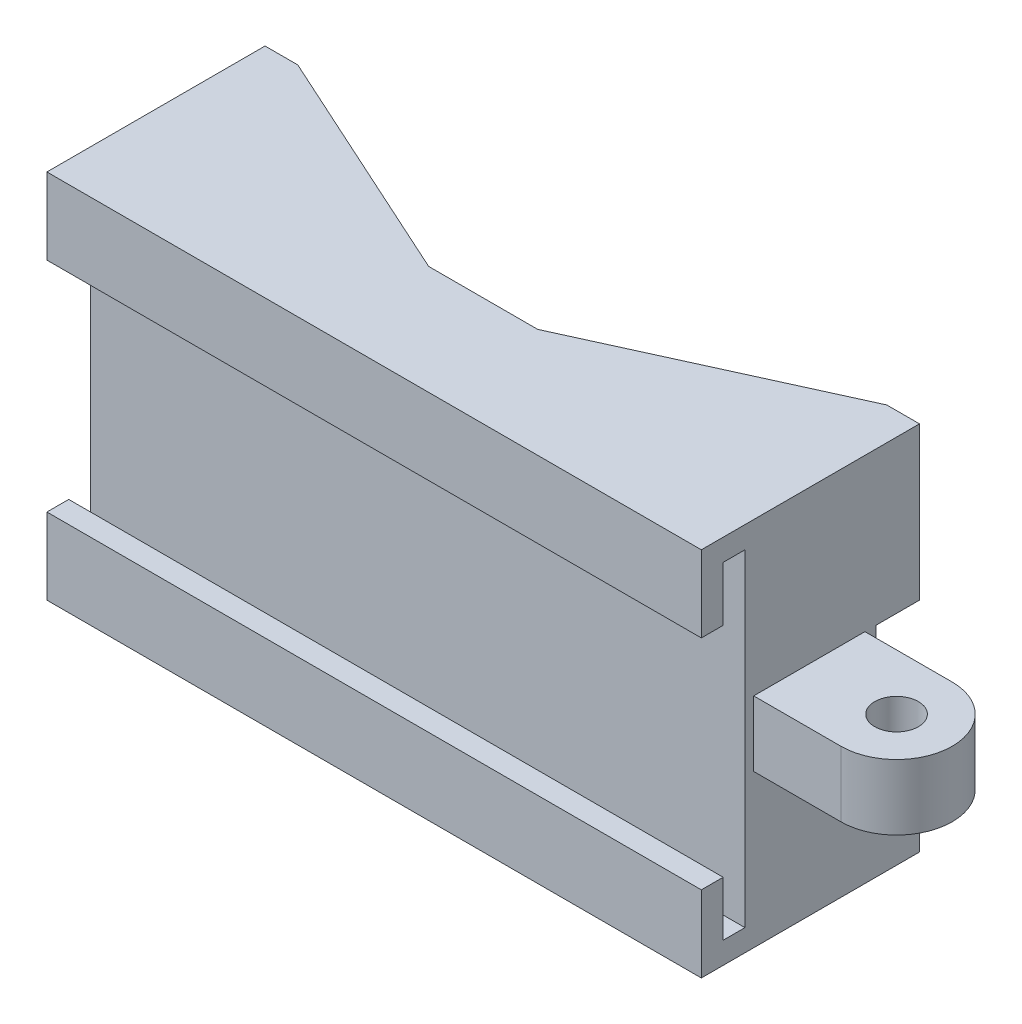
from build123d import *

# Parameters (mm, degrees)
SKETCH1_W           = 300
SKETCH1_H           = 170
BOSS_EXTRUDE1_DEPTH = 10
SKETCH2_W           = 300
SKETCH2_H           = 10
BOSS_EXTRUDE2_DEPTH = 20
SKETCH4_W           = 300
SKETCH4_H           = 10
BOSS_EXTRUDE3_DEPTH = 25
BOSS_EXTRUDE4_DEPTH = 85
CUT_EXTRUDE1_DEPTH  = 15
SKETCH8_R           = 10
BOSS_EXTRUDE5_DEPTH = 15


with BuildPart() as part:
    # Sketch1 → Boss-Extrude1 (new body)
    with BuildSketch(Plane.XY):
        Rectangle(SKETCH1_W, SKETCH1_H)
    extrude(amount=BOSS_EXTRUDE1_DEPTH)

    # Sketch2 → Boss-Extrude2 (add)
    with BuildSketch(Plane.XY.offset(10)):
        with Locations((0, 80)):
            Rectangle(SKETCH2_W, SKETCH2_H)
        with Locations((0, -80)):
            Rectangle(SKETCH2_W, SKETCH2_H)
    extrude(amount=BOSS_EXTRUDE2_DEPTH)

    # Sketch4 → Boss-Extrude3 (add)
    with BuildSketch(Plane.XZ.offset(-75)):
        with Locations((0, 25)):
            Rectangle(SKETCH4_W, SKETCH4_H)
    boss_extrude3 = extrude(amount=BOSS_EXTRUDE3_DEPTH)

    # Mirror1: Boss-Extrude3 across plane
    add(boss_extrude3.mirror(Plane.ZX))

    # Sketch5 → Boss-Extrude4 (add, symmetric)
    with BuildSketch(Plane(origin=(0, 0, 0), x_dir=(1, 0, 0), z_dir=(0, 1, 0))):
        Polygon((-150, 0), (-150, 70), (-135, 70), (-25, 20), (0, 20), (0, 0), align=None)
    boss_extrude4 = extrude(amount=BOSS_EXTRUDE4_DEPTH, both=True)

    # Sketch6 → Cut-Extrude1 (cut, symmetric)
    with BuildSketch(Plane(origin=(0, 0, 0), x_dir=(1, 0, 0), z_dir=(0, 1, 0))):
        Polygon((-150, 70), (-135, 70), (-25, 20), (0, 20), (0, 0), (-25, 0), (-135, 50), (-150, 50), align=None)
    cut_extrude1 = extrude(amount=CUT_EXTRUDE1_DEPTH, both=True, mode=Mode.SUBTRACT)

    # Mirror2: Boss-Extrude4, Cut-Extrude1 across plane
    add(boss_extrude4.mirror(Plane(origin=(0, 0, 0), x_dir=(0, 0, 1), z_dir=(1, 0, 0))))
    add(cut_extrude1.mirror(Plane(origin=(0, 0, 0), x_dir=(0, 0, 1), z_dir=(1, 0, 0))), mode=Mode.SUBTRACT)

    # Sketch8 → Boss-Extrude5 (add, symmetric)
    with BuildSketch(Plane(origin=(0, 0, 0), x_dir=(1, 0, 0), z_dir=(0, 1, 0))):
        with BuildLine():
            Line((150, -6), (190, -6))
            ThreePointArc((190, -6), (215.5, 19.5), (190, 45))
            Line((190, 45), (150, 45))
            Line((150, 45), (150, -6))
        make_face()
        with Locations(Location((190, 19.5, 0), (0, 0, 270))):
            Circle(SKETCH8_R, mode=Mode.SUBTRACT)
    extrude(amount=BOSS_EXTRUDE5_DEPTH, both=True)


solid = part.part
